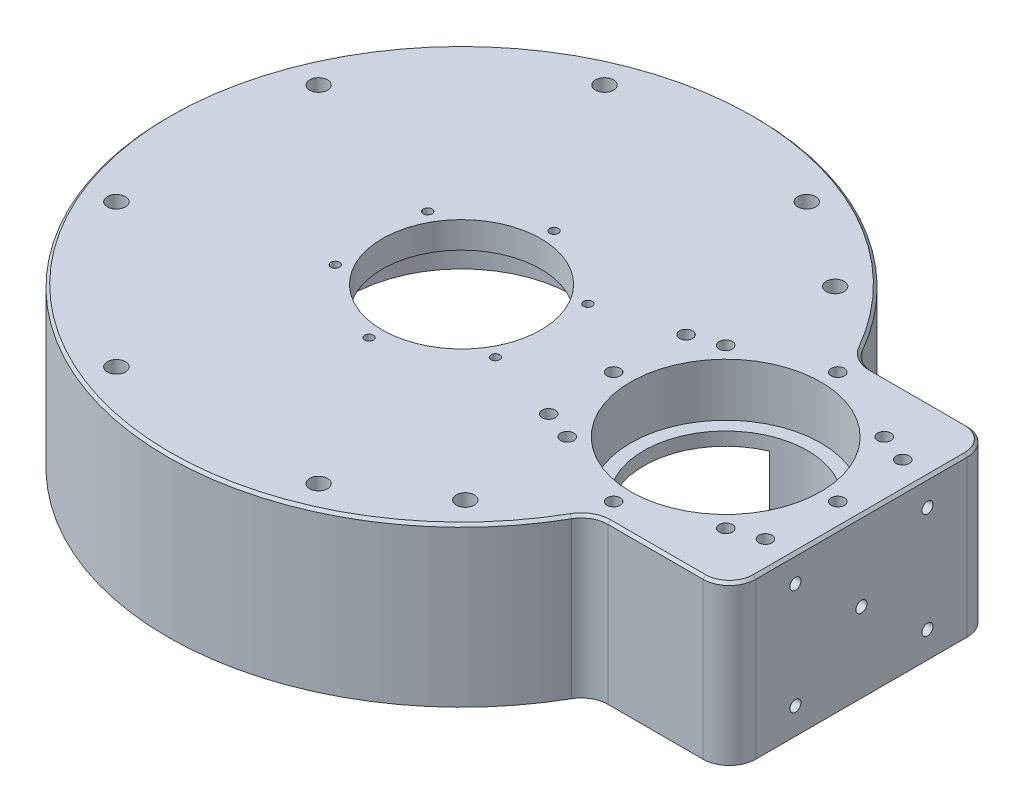
SolidWorks part; units mm, degrees
material "6061Al"
ref_plane "前视基准面" through (0, 0, 0) normal (0, 0, 1) x (1, 0, 0)
ref_plane "上视基准面" through (0, 0, 0) normal (0, 1, 0) x (1, 0, 0)
ref_plane "右视基准面" through (0, 0, 0) normal (1, 0, 0) x (0, 0, -1)
sketch "草图1" plane through (0, 0, 0) normal (0, 0, 1) x (1, 0, 0)
  line L0 (92.5, 0) -> (111.25, 0)
  line L2 (39.5, 60) -> (111.25, 60)
  line L3 (92.5, 35) -> (42.5, 35)
  line L5 (42.5, 35) -> (42.5, 45)
  line L6 (42.5, 45) -> (39.5, 45)
  line L8 (39.5, 45) -> (39.5, 60)
  line L9 (111.25, 60) -> (111.25, 0)
  line L10 (92.5, 35) -> (92.5, 0)
  line L13 (0, 0) -> (0, 181.0754) construction
  line L14 (-82.25, 0) -> (82.25, 0) construction
  dimension "D1" = 60
  dimension "D2" = 3
  dimension "D3" = 35
  dimension "D4" = 185
  dimension "D5" = 45
  dimension "D6" = 85
  dimension "D7" = 222.5
revolve "旋转1" add sketch "草图1" angle 360 about L13
sketch "草图2" plane through (0, 0, 0) normal (0, -1, 0) x (1, 0, 0)
  line L0 (0, 0) -> (111.25, 0) construction
  line L2 (99.3809, 50) -> (151.3809, 50)
  line L3 (99.3809, 50) -> (99.3809, -50)
  line L4 (99.3809, -50) -> (151.3809, -50)
  line L5 (151.3809, 50) -> (151.3809, -50)
  circle A0 centre (0, 0) radius 111.25 construction
  dimension "D1" = 100
  dimension "D2" = 52
extrude "凸台-拉伸1" add sketch "草图2" against normal through all
sketch "草图3" plane through (0, 60, 0) normal (0, 1, 0) x (1, 0, 0)
  circle A0 centre (100, 0) radius 36
  dimension "D1" = 72
  dimension "D2" = 100
extrude "切除-拉伸1" cut sketch "草图3" against normal offset from surface (20 mm away) 40
sketch "草图4" plane through (0, 40, 0) normal (0, 1, 0) x (1, 0, 0)
  circle A2 centre (100, 0) radius 31
  circle A3 centre (100, 0) radius 31
  dimension "D1" = 5
extrude "切除-拉伸2" cut sketch "草图4" against normal offset from surface (24 mm away) 16
sketch "草图9" plane through (0, 16, 0) normal (0, 1, 0) x (1, 0, 0)
  circle A0 centre (0, 0) radius 92.5 construction
  circle A1 centre (0, 0) radius 92.5
  circle A2 centre (0, 0) radius 95.5
  dimension "D1" = 3
extrude "凸台-拉伸2" add sketch "草图9" along normal blind 3
hole_wizard "M8 螺纹孔3" positions "草图11" profile "草图12" tap size "M8" standard "ISO"
sketch "草图11" plane through (0, 0, 0) normal (0, -1, 0) x (-1, 0, 0)
  line L1 (0, 0) -> (39.7991, 96.0835) construction
  line L2 (0, 0) -> (0, 142.126) construction
  point P28 (39.7991, 96.0835)
  point P42 (96.0835, 39.7991)
  point P43 (96.0835, -39.7991)
  point P44 (39.7991, -96.0835)
  point P45 (-39.7991, -96.0835)
  point P46 (-96.0835, -39.7991)
  point P47 (-96.0835, 39.7991)
  point P48 (-39.7991, 96.0835)
  dimension "D1" = 8
  dimension "D2" = 104
cosmetic thread "孔螺蚊线20" parameters "D2"=8
cosmetic thread "孔螺蚊线21" parameters "D2"=8
cosmetic thread "孔螺蚊线22" parameters "D2"=8
cosmetic thread "孔螺蚊线23" parameters "D2"=8
cosmetic thread "孔螺蚊线24" parameters "D2"=8
cosmetic thread "孔螺蚊线25" parameters "D2"=8
cosmetic thread "孔螺蚊线26" parameters "D2"=8
cosmetic thread "孔螺蚊线27" parameters "D2"=8
sketch "草图12" plane through (-39.7991, 0, -96.0835) normal (1, 0, 0) x (0, 0, -1)
  line L0 (0, 0) -> (0, 21.7929)
  line L1 (0, 21.7929) -> (3.4, 19.75)
  line L2 (3.4, 19.75) -> (3.4, 0)
  line L5 (3.4, 0) -> (0, 0)
  line L10 (0, 21.7929) -> (-3.4, 19.75) construction
  line L11 (0, -6.35) -> (0, 107.95) construction
  dimension "螺纹孔钻头直径" = 6.8
  dimension "螺纹孔钻头深度" = 19.75
  dimension "导头角度" = 118
hole_wizard "M6 螺纹孔1" positions "草图15" profile "草图16" tap size "M6" standard "ISO"
sketch "草图15" plane through (0, 60, 0) normal (0, 1, 0) x (1, 0, 0)
  line L1 (70, -30) -> (130, -30)
  line L2 (70, -30) -> (70, 30)
  line L3 (70, 30) -> (130, 30)
  line L4 (130, -30) -> (130, 30)
  line L5 (70, -30) -> (130, 30) construction
  line L6 (70, 30) -> (130, -30) construction
  circle A0 centre (100, 0) radius 42.4264
  point P0 (70, 30)
  point P2 (130, 30)
  point P4 (130, -30)
  point P6 (70, -30)
  point P9 (100, 0)
  point P52 (100, 42.4264)
  point P54 (100, -42.4264)
  point P57 (57.5736, 0)
  point P64 (142.4264, 0)
  point P65 (59, -26)
  point P68 (59, 26)
  point P71 (141, 26)
  point P74 (141, -26)
  dimension "D1" = 60
sketch "草图16" plane through (70, 60, -30) normal (1, 0, 0) x (0, 0, 1)
  line L0 (0, 0) -> (0, 16.5022)
  line L1 (0, 16.5022) -> (2.5, 15)
  line L2 (2.5, 15) -> (2.5, 0)
  line L5 (2.5, 0) -> (0, 0)
  line L10 (0, 16.5022) -> (-2.5, 15) construction
  line L11 (0, -6.35) -> (0, 107.95) construction
  dimension "螺纹孔钻头直径" = 5
  dimension "螺纹孔钻头深度" = 15
  dimension "导头角度" = 118
cosmetic thread "孔螺蚊线16" parameters "D1"=12, "D2"=6
cosmetic thread "孔螺蚊线17" parameters "D1"=12, "D2"=6
cosmetic thread "孔螺蚊线18" parameters "D1"=12, "D2"=6
cosmetic thread "孔螺蚊线19" parameters "D1"=12, "D2"=6
cosmetic thread "孔螺蚊线34" parameters "D1"=12, "D2"=6
cosmetic thread "孔螺蚊线35" parameters "D1"=12, "D2"=6
cosmetic thread "孔螺蚊线37" parameters "D1"=12, "D2"=6
cosmetic thread "孔螺蚊线38" parameters "D1"=12, "D2"=6
cosmetic thread "孔螺蚊线49" parameters "D1"=12, "D2"=6
cosmetic thread "孔螺蚊线50" parameters "D1"=12, "D2"=6
cosmetic thread "孔螺蚊线51" parameters "D1"=12, "D2"=6
cosmetic thread "孔螺蚊线52" parameters "D1"=12, "D2"=6
sketch "草图17" plane through (0, 19, 0) normal (0, 1, 0) x (1, 0, 0)
  arc A4 (87.9762, -28.5732) -> (90.7962, -29.6022) centre (100, 0) ccw
  arc A5 (90.7962, -29.6022) -> (90.7963, 29.6022) centre (0, 0) ccw
  arc A6 (90.7963, 29.6022) -> (87.9762, 28.5732) centre (100, 0) ccw
  arc A7 (87.9762, -28.5732) -> (87.9762, 28.5732) centre (0, 0) ccw
  arc A8 (87.9762, -28.5732) -> (90.7962, -29.6022) centre (100, 0) ccw
  arc A9 (90.7962, -29.6022) -> (90.7963, 29.6022) centre (0, 0) ccw
  arc A10 (90.7963, 29.6022) -> (87.9762, 28.5732) centre (100, 0) ccw
  arc A11 (87.9762, -28.5732) -> (87.9762, 28.5732) centre (0, 0) ccw
  dimension "D1" = 0
extrude "切除-拉伸4" cut sketch "草图17" against normal up to surface (3 mm away) up to face at (113.25, 16, 0)
sketch "草图18" plane through (0, 60, 0) normal (0, 1, 0) x (1, 0, 0)
  circle A0 centre (0, 0) radius 39.5 construction
  circle A1 centre (0, 0) radius 39.5
  circle A2 centre (0, 0) radius 30
  dimension "D1" = 60
extrude "凸台-拉伸3" add sketch "草图18" against normal blind 10
hole_wizard "M4 螺纹孔1" positions "草图19" profile "草图20" tap size "M4" standard "ISO"
sketch "草图19" plane through (0, 60, 0) normal (0, 1, 0) x (1, 0, 0)
  line L0 (0, 0) -> (0, 35) construction
  circle A3 centre (0, 0) radius 35
  circle A4 centre (0, 0) radius 35
  point P0 (0, 35)
  point P17 (30.3109, 17.5)
  point P18 (30.3109, -17.5)
  point P19 (0, -35)
  point P20 (-30.3109, -17.5)
  point P21 (-30.3109, 17.5)
  dimension "D1" = 5
  dimension "D2" = 6
cosmetic thread "孔螺蚊线28" parameters "D1"=8, "D2"=4
cosmetic thread "孔螺蚊线29" parameters "D1"=8, "D2"=4
cosmetic thread "孔螺蚊线30" parameters "D1"=8, "D2"=4
cosmetic thread "孔螺蚊线31" parameters "D1"=8, "D2"=4
cosmetic thread "孔螺蚊线32" parameters "D1"=8, "D2"=4
cosmetic thread "孔螺蚊线33" parameters "D1"=8, "D2"=4
sketch "草图20" plane through (0, 60, -35) normal (1, 0, 0) x (0, 0, 1)
  line L0 (0, 0) -> (0, 8.9914)
  line L1 (0, 8.9914) -> (1.65, 8)
  line L2 (1.65, 8) -> (1.65, 0)
  line L5 (1.65, 0) -> (0, 0)
  line L10 (0, 8.9914) -> (-1.65, 8) construction
  line L11 (0, -6.35) -> (0, 107.95) construction
  dimension "螺纹孔钻头直径" = 3.3
  dimension "螺纹孔钻头深度" = 8
  dimension "导头角度" = 118
hole_wizard "M8 螺纹孔5" positions "草图21" profile "草图22" tap size "M8" standard "ISO"
sketch "草图21" plane through (0, 60, 0) normal (0, 1, 0) x (1, 0, 0)
  line L0 (0, 0) -> (38.2683, 92.388) construction
  line L1 (0, 0) -> (151.3809, 0) construction
  line L2 (151.3809, 50) -> (151.3809, -50) construction
  point P0 (38.2683, 92.388)
  point P8 (38.2683, -92.388)
  point P9 (-38.2683, -92.388)
  point P10 (-92.388, -38.2683)
  point P11 (-92.388, 38.2683)
  point P12 (-38.2683, 92.388)
  point P29 (92.388, -38.2683) [skipped]
  point P30 (92.388, 38.2683) [skipped]
  point P32 (71.4143, 70)
  point P35 (71.4143, -70)
  dimension "D2" = 100
  dimension "D1" = 8
sketch "草图22" plane through (38.2683, 60, -92.388) normal (1, 0, 0) x (0, 0, 1)
  line L0 (0, 0) -> (0, 21.7929)
  line L1 (0, 21.7929) -> (3.4, 19.75)
  line L2 (3.4, 19.75) -> (3.4, 0)
  line L5 (3.4, 0) -> (0, 0)
  line L10 (0, 21.7929) -> (-3.4, 19.75) construction
  line L11 (0, -6.35) -> (0, 107.95) construction
  dimension "螺纹孔钻头直径" = 6.8
  dimension "螺纹孔钻头深度" = 19.75
  dimension "导头角度" = 118
cosmetic thread "孔螺蚊线39" parameters "D1"=16, "D2"=8
cosmetic thread "孔螺蚊线40" parameters "D1"=16, "D2"=8
cosmetic thread "孔螺蚊线41" parameters "D1"=16, "D2"=8
cosmetic thread "孔螺蚊线42" parameters "D1"=16, "D2"=8
cosmetic thread "孔螺蚊线43" parameters "D1"=16, "D2"=8
cosmetic thread "孔螺蚊线46" parameters "D1"=16, "D2"=8
cosmetic thread "孔螺蚊线47" parameters "D1"=16, "D2"=8
cosmetic thread "孔螺蚊线48" parameters "D1"=16, "D2"=8
fillet "圆角1" radius 10 4 edges at (99.3809, 30, 50) (99.3809, 30, -50) (151.3809, 30, -50) (151.3809, 30, 50)
chamfer "倒角1" distance 1 angle 45 8 edges at (148.452, 60, 47.0711) (148.452, 60, -47.0711) (123.3724, 60, 50) (123.3724, 60, -50) (100.3382, 60, 51.3546) (100.3382, 60, -51.3546) (-111.25, 60, 0) (151.3809, 60, 0)
hole_wizard "M5 螺纹孔1" positions "草图25" profile "草图24" tap size "M5" standard "ISO"
sketch "草图25" plane through (151.3809, 0, 0) normal (1, 0, 0) x (0, 0, -1)
  line L0 (0, 60) -> (0, 0)
  line L1 (-40, 60) -> (40, 60) construction
  line L4 (-25, 10) -> (25, 10)
  line L5 (-25, 10) -> (-25, 50)
  line L6 (-25, 50) -> (25, 50)
  line L7 (25, 10) -> (25, 50)
  line L8 (-25, 10) -> (25, 50) construction
  line L9 (-25, 50) -> (25, 10) construction
  point P0 (-25, 50)
  point P10 (0, 30)
  point P11 (25, 50)
  point P14 (-25, 10)
  point P16 (25, 10)
  dimension "D1" = 50
  dimension "D2" = 40
sketch "草图24" plane through (151.3809, 50, 25) normal (0, 1, 0) x (0, 0, -1)
  line L0 (0, 0) -> (0, 13.6618)
  line L1 (0, 13.6618) -> (2.1, 12.4)
  line L2 (2.1, 12.4) -> (2.1, 0)
  line L5 (2.1, 0) -> (0, 0)
  line L10 (0, 13.6618) -> (-2.1, 12.4) construction
  line L11 (0, -6.35) -> (0, 107.95) construction
  dimension "螺纹孔钻头直径" = 4.2
  dimension "螺纹孔钻头深度" = 12.4
  dimension "导头角度" = 118
